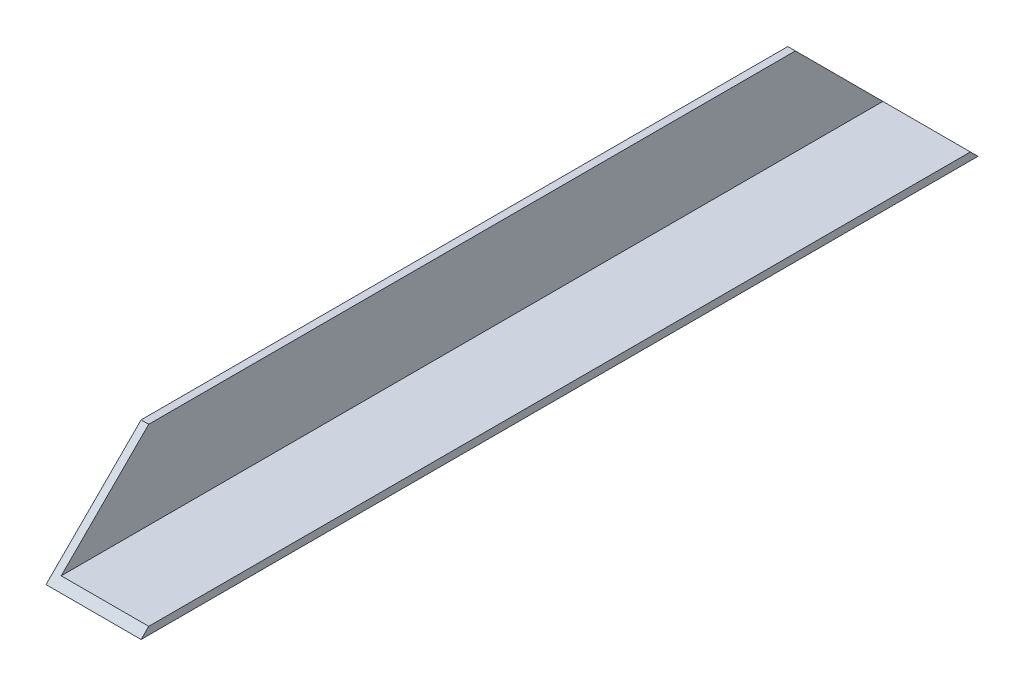
from build123d import *

# Parameters (mm, degrees)
EXTRUDE_1_DEPTH     = 550
CUT_EXTRUDE_1_DEPTH = 578.711000415


with BuildPart() as part:
    # 草图1 → 凸台-拉伸1 (new, symmetric)
    with BuildSketch(Plane.XY):
        Polygon((0, 125), (10, 125), (10, 10), (125, 10), (125, 0), (0, 0), align=None)
    extrude(amount=EXTRUDE_1_DEPTH, both=True)

    # 草图2 → 切除-拉伸1 (cut, through all)
    with BuildSketch(Plane(origin=(125, 0, 0), x_dir=(0, 0, -1), z_dir=(1, 0, 0))):
        Polygon((-550, 0), (-550, 125), (-425, 125), align=None)
        Polygon((425, 125), (550, 0), (550, 125), align=None)
    extrude(amount=-CUT_EXTRUDE_1_DEPTH, mode=Mode.SUBTRACT)


solid = part.part
